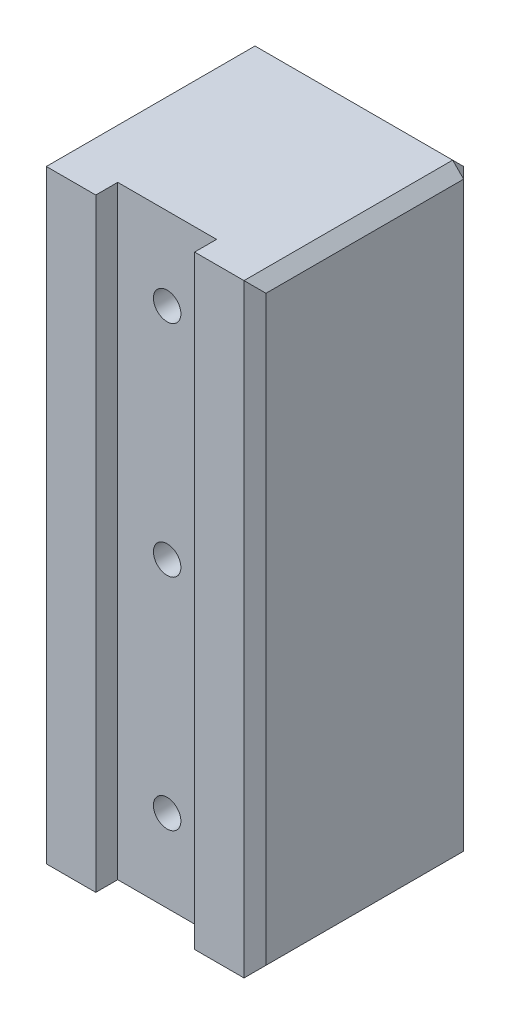
from build123d import *

# Parameters (mm, degrees)
SKETCH1_W             = 20
SKETCH1_H             = 55
BOSS_EXTRUDE1_DEPTH   = 20
SKETCH2_W             = 9
SKETCH2_H             = 55
CUT_EXTRUDE1_DEPTH    = 2
M3_TAPPED_HOLE1_D     = 2.5
M3_TAPPED_HOLE1_DEPTH = 7.5
M3_TAPPED_HOLE1_TIP   = 0.751075774
M4_TAPPED_HOLE1_D     = 3.3
M4_TAPPED_HOLE1_DEPTH = 10.1
M4_TAPPED_HOLE1_TIP   = 0.991420021
M5_TAPPED_HOLE1_D     = 4.2
M5_TAPPED_HOLE1_DEPTH = 12.4
M5_TAPPED_HOLE1_TIP   = 1.2618073
CHAMFER1_SIZE         = 1


with BuildPart() as part:
    # Sketch1 → Boss-Extrude1 (new body)
    with BuildSketch(Plane.XY):
        Rectangle(SKETCH1_W, SKETCH1_H)
    extrude(amount=BOSS_EXTRUDE1_DEPTH)

    # Sketch2 → Cut-Extrude1 (cut)
    with BuildSketch(Plane.XY.offset(20)):
        Rectangle(SKETCH2_W, SKETCH2_H)
    extrude(amount=-CUT_EXTRUDE1_DEPTH, mode=Mode.SUBTRACT)

    # M3 Tapped Hole1
    with Locations(Plane.XY.offset(18)):
        with Locations((0, 20), (0, 0), (0, -20)):
            Hole(M3_TAPPED_HOLE1_D / 2, depth=M3_TAPPED_HOLE1_DEPTH)
            with Locations((0, 0, -(M3_TAPPED_HOLE1_DEPTH + M3_TAPPED_HOLE1_TIP / 2))):  # 118° drill point
                Cone(0, M3_TAPPED_HOLE1_D / 2, M3_TAPPED_HOLE1_TIP, mode=Mode.SUBTRACT)

    # M4 Tapped Hole1
    with Locations(Plane(origin=(0, -27.5, 0), x_dir=(-1, 0, 0), z_dir=(0, -1, 0))):
        with Locations((0, -13), (0, -5.5)):
            Hole(M4_TAPPED_HOLE1_D / 2, depth=M4_TAPPED_HOLE1_DEPTH)
            with Locations((0, 0, -(M4_TAPPED_HOLE1_DEPTH + M4_TAPPED_HOLE1_TIP / 2))):  # 118° drill point
                Cone(0, M4_TAPPED_HOLE1_D / 2, M4_TAPPED_HOLE1_TIP, mode=Mode.SUBTRACT)

    # M5 Tapped Hole1
    with Locations(Plane(origin=(0, 0, 0), x_dir=(-1, 0, 0), z_dir=(0, 0, -1))):
        with Locations((0, 20), (0, -20)):
            Hole(M5_TAPPED_HOLE1_D / 2, depth=M5_TAPPED_HOLE1_DEPTH)
            with Locations((0, 0, -(M5_TAPPED_HOLE1_DEPTH + M5_TAPPED_HOLE1_TIP / 2))):  # 118° drill point
                Cone(0, M5_TAPPED_HOLE1_D / 2, M5_TAPPED_HOLE1_TIP, mode=Mode.SUBTRACT)

    # Chamfer1
    chamfer1_edges = [part.edges().sort_by_distance(p)[0] for p in [
        (-10, 0, 20),
        (10, 0, 20),
        (0, -27.5, 0),
        (-10, 0, 0),
        (0, 27.5, 0),
        (10, 0, 0),
        (10, -27.5, 10),
        (-10, -27.5, 10),
        (-10, 27.5, 10),
        (10, 27.5, 10),
    ]]
    chamfer(chamfer1_edges, length=CHAMFER1_SIZE)


solid = part.part
